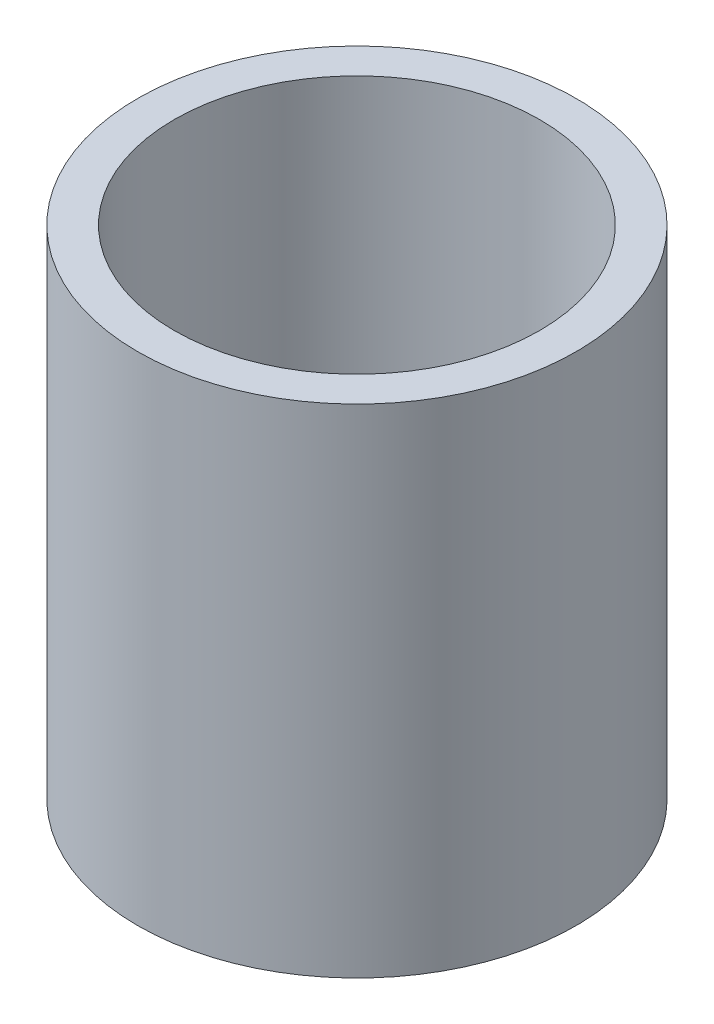
SolidWorks part; units mm, degrees
ref_plane "前视基准面" through (0, 0, 0) normal (0, 0, 1) x (1, 0, 0)
ref_plane "上视基准面" through (0, 0, 0) normal (0, 1, 0) x (1, 0, 0)
ref_plane "右视基准面" through (0, 0, 0) normal (1, 0, 0) x (0, 0, -1)
sketch "草图1" plane through (0, 0, 0) normal (0, 1, 0) x (1, 0, 0)
  circle A0 centre (0, 0) radius 12.5
  circle A1 centre (0, 0) radius 15
  dimension "D1" = 25
  dimension "D2" = 30
extrude "凸台-拉伸1" add sketch "草图1" along normal blind 34
